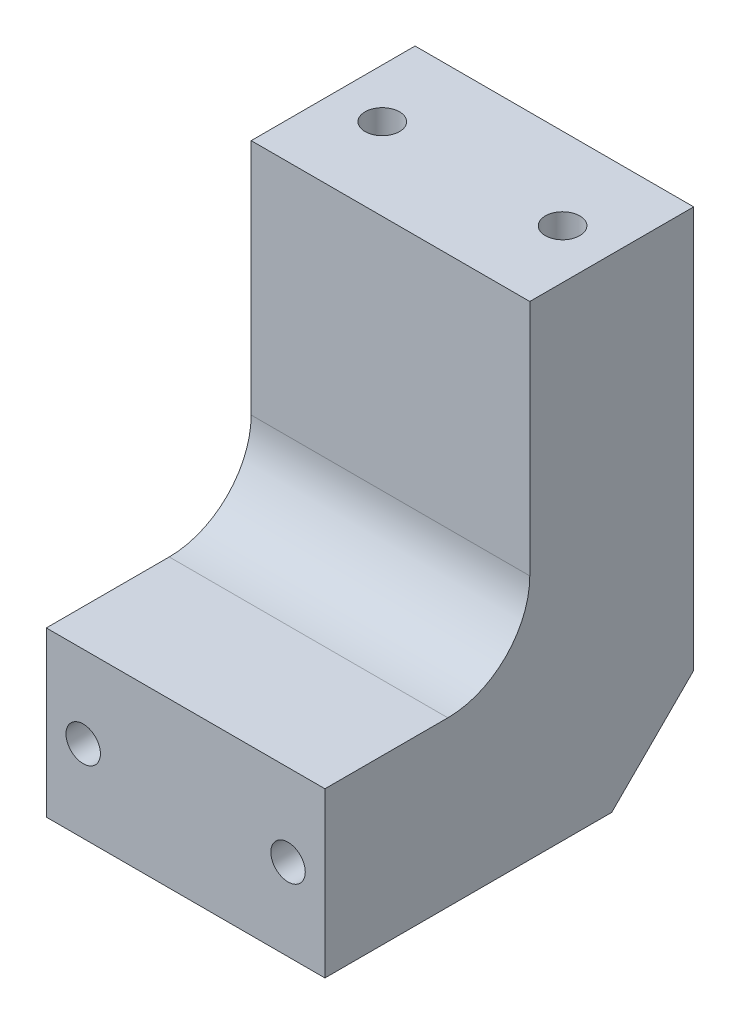
from build123d import *

# Parameters (mm, degrees)
SKETCH1_W             = 34
SKETCH1_H             = 45
BOSS_EXTRUDE1_DEPTH   = 59
SKETCH2_W             = 25
SKETCH2_H             = 39
CUT_EXTRUDE1_DEPTH    = 45
CHAMFER1_SIZE         = 10
FILLET1_R             = 10
M5_TAPPED_HOLE1_D     = 4.2
M5_TAPPED_HOLE1_DEPTH = 12.4
M5_TAPPED_HOLE1_TIP   = 1.2618073
M5_TAPPED_HOLE2_D     = 4.2
M5_TAPPED_HOLE2_DEPTH = 12.4
M5_TAPPED_HOLE2_TIP   = 1.2618073


with BuildPart() as part:
    # Sketch1 → Boss-Extrude1 (new body)
    with BuildSketch(Plane(origin=(0, 0, 0), x_dir=(1, 0, 0), z_dir=(0, 1, 0))):
        Rectangle(SKETCH1_W, SKETCH1_H)
    extrude(amount=BOSS_EXTRUDE1_DEPTH)

    # Sketch2 → Cut-Extrude1 (cut)
    with BuildSketch(Plane(origin=(17, 0, 0), x_dir=(0, 0, -1), z_dir=(1, 0, 0))):
        with Locations((-10, 39.5)):
            Rectangle(SKETCH2_W, SKETCH2_H)
    extrude(amount=-CUT_EXTRUDE1_DEPTH, mode=Mode.SUBTRACT)

    # Chamfer1
    chamfer1_edges = [part.edges().sort_by_distance(p)[0] for p in [
        (0, 0, -22.5),
    ]]
    chamfer(chamfer1_edges, length=CHAMFER1_SIZE)

    # Fillet1
    fillet1_edges = [part.edges().sort_by_distance(p)[0] for p in [
        (0, 20, -2.5),
    ]]
    fillet(fillet1_edges, radius=FILLET1_R)

    # M5 Tapped Hole1
    with Locations(Plane(origin=(-11, 59, -12.5), x_dir=(0, 0, 1), z_dir=(0, 1, 0))):
        with Locations((0, 0), (0, 22)):
            Hole(M5_TAPPED_HOLE1_D / 2, depth=M5_TAPPED_HOLE1_DEPTH)
            with Locations((0, 0, -(M5_TAPPED_HOLE1_DEPTH + M5_TAPPED_HOLE1_TIP / 2))):  # 118° drill point
                Cone(0, M5_TAPPED_HOLE1_D / 2, M5_TAPPED_HOLE1_TIP, mode=Mode.SUBTRACT)

    # M5 Tapped Hole2
    with Locations(Plane(origin=(-12.5, 10, 22.5), x_dir=(1, 0, 0), z_dir=(0, 0, 1))):
        with Locations((0, 0), (25, 0)):
            Hole(M5_TAPPED_HOLE2_D / 2, depth=M5_TAPPED_HOLE2_DEPTH)
            with Locations((0, 0, -(M5_TAPPED_HOLE2_DEPTH + M5_TAPPED_HOLE2_TIP / 2))):  # 118° drill point
                Cone(0, M5_TAPPED_HOLE2_D / 2, M5_TAPPED_HOLE2_TIP, mode=Mode.SUBTRACT)


solid = part.part
